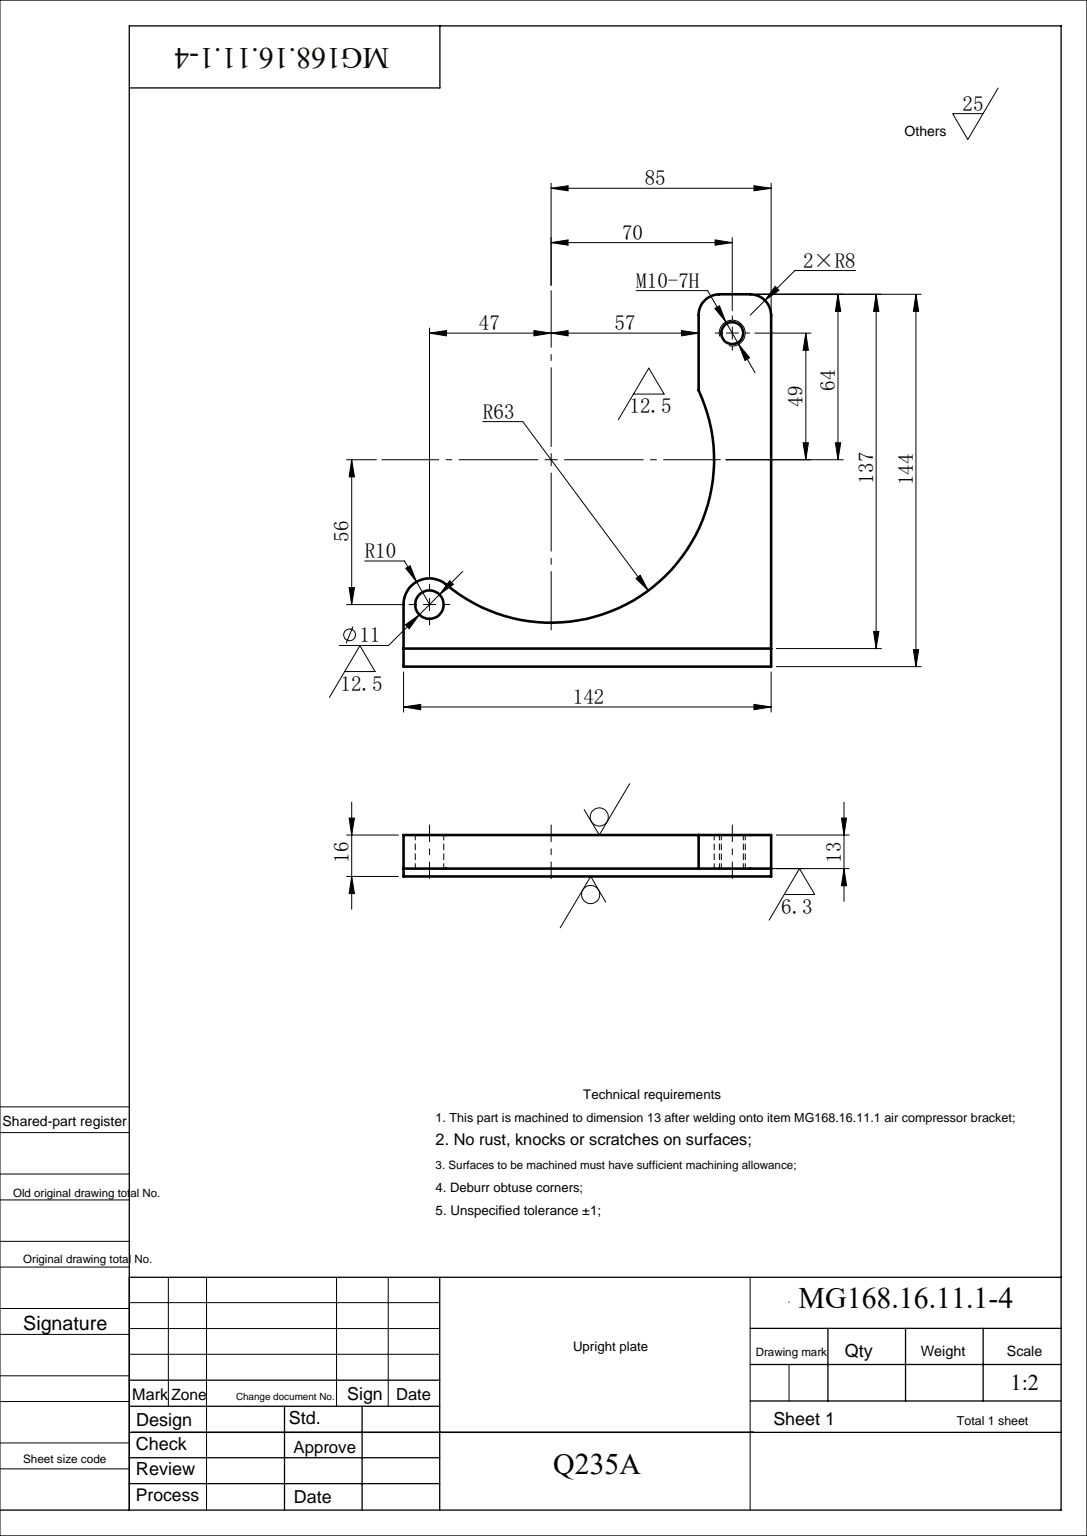
from build123d import *

# Parameters (mm, degrees)
SKETCH1_R           = 5.5
BOSS_EXTRUDE1_DEPTH = 6.5
SKETCH2_W           = 142
SKETCH2_H           = 7
BOSS_EXTRUDE2_DEPTH = 3
M10_TAPPED_HOLE1_D  = 8.5
FILLET1_R           = 8


with BuildPart() as part:
    # Sketch1 → Boss-Extrude1 (new, symmetric)
    with BuildSketch(Plane.XY):
        with BuildLine():
            Line((28, 144), (28, 106.83281573))
            ThreePointArc((28, 106.83281573), (46.591206617, 30.06239302), (125.561643836, 31.794678205))
            ThreePointArc((125.561643836, 31.794678205), (136.219978576, 33.209008103), (142, 24.143039825))
            Line((142, 24.143039825), (142, 0))
            Line((142, 0), (0, 0))
            Line((0, 0), (0, 144))
            Line((0, 144), (28, 144))
        make_face()
        with Locations(Location((132, 24, 0), (0, 0, 180))):
            Circle(SKETCH1_R, mode=Mode.SUBTRACT)
    extrude(amount=BOSS_EXTRUDE1_DEPTH, both=True)

    # Sketch2 → Boss-Extrude2 (add)
    with BuildSketch(Plane.XY.offset(-6.5)):
        with Locations((71, 3.5)):
            Rectangle(SKETCH2_W, SKETCH2_H)
    extrude(amount=-BOSS_EXTRUDE2_DEPTH)

    # M10 Tapped Hole1 (through all)
    with Locations(Plane.XY.offset(6.5)):
        with Locations((15, 129)):
            Hole(M10_TAPPED_HOLE1_D / 2)

    # Fillet1
    fillet1_edges = [part.edges().sort_by_distance(p)[0] for p in [
        (0, 144, 0),
        (28, 144, 0),
    ]]
    fillet(fillet1_edges, radius=FILLET1_R)


solid = part.part
